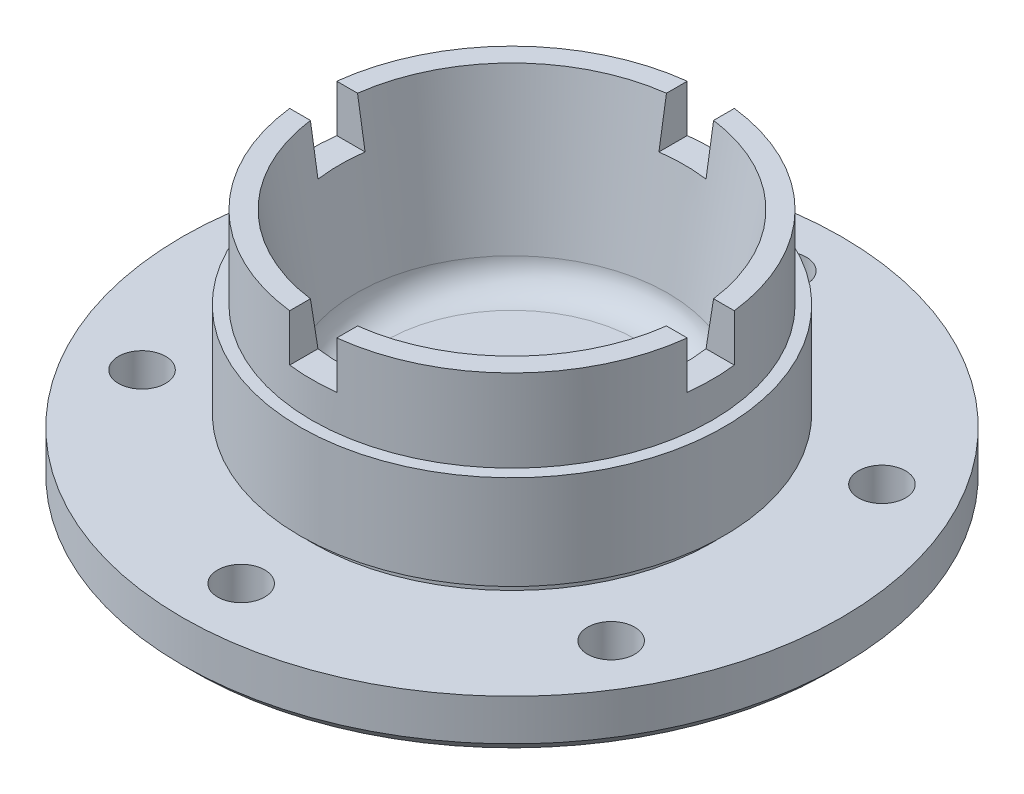
from build123d import *

# Parameters (mm, degrees)
SKETCH2_W          = 33.532576539
SKETCH2_H          = 8
SKETCH2_W_2        = 8
SKETCH2_H_2        = 33.532576539
CUT_EXTRUDE1_DEPTH = 8
SKETCH3_R          = 4
CUT_EXTRUDE2_DEPTH = 93
SCALE_1_SCALE      = 1.875


with BuildPart() as part:
    # Sketch1 → Revolve1 (revolve)
    with BuildSketch(Plane.XY, mode=Mode.PRIVATE) as revolve1_sk:
        with BuildLine():
            Line((0, 11), (0, 2))
            Line((0, 2), (31, 2))
            Line((31, 2), (32, 0))
            Line((32, 0), (54, 0))
            Line((54, 0), (56, 2))
            Line((56, 2), (56, 9))
            Line((56, 9), (34, 9))
            Line((34, 9), (34, 11))
            Line((34, 11), (36, 11))
            Line((36, 11), (36, 27))
            Line((36, 27), (34, 27))
            Line((34, 27), (34, 41))
            Line((34, 41), (30.5, 41))
            Line((30.5, 41), (26.45024814, 15.502481405))
            ThreePointArc((26.45024814, 15.502481405), (24.830088793, 12.292737332), (21.475062189, 11))
            Line((21.475062189, 11), (16.570568921, 11))
            Line((16.570568921, 11), (0, 11))
        make_face()
    revolve(revolve1_sk.sketch.rotate(Axis((0, 2, 0), (0, 1, 0)), 90), axis=Axis((0, 2, 0), (0, 1, 0)))

    # Sketch2 → Cut-Extrude1 (cut)
    with BuildSketch(Plane(origin=(0, 41, 0), x_dir=(1, 0, 0), z_dir=(0, 1, 0))):
        with Locations((31.449191607, 0)):
            Rectangle(SKETCH2_W, SKETCH2_H)
        with Locations((0, 31.449191607)):
            Rectangle(SKETCH2_W_2, SKETCH2_H_2)
        with Locations((0, -31.449191607)):
            Rectangle(SKETCH2_W_2, SKETCH2_H_2)
        with Locations((-31.449191607, 0)):
            Rectangle(SKETCH2_W, SKETCH2_H)
    extrude(amount=-CUT_EXTRUDE1_DEPTH, mode=Mode.SUBTRACT)

    # Sketch3 → Cut-Extrude2 (cut)
    with BuildSketch(Plane(origin=(0, 41, 0), x_dir=(1, 0, 0), z_dir=(0, 1, 0))):
        with Locations(Location((-39.837168574, -23, 0), (0, 0, 270))):
            Circle(SKETCH3_R)
        with Locations(Location((0, 46, 0), (0, 0, 270))):
            Circle(SKETCH3_R)
        with Locations(Location((39.837168574, 23, 0), (0, 0, 270))):
            Circle(SKETCH3_R)
        with Locations(Location((-39.837168574, 23, 0), (0, 0, 270))):
            Circle(SKETCH3_R)
        with Locations(Location((0, -46, 0), (0, 0, 270))):
            Circle(SKETCH3_R)
        with Locations(Location((39.837168574, -23, 0), (0, 0, 270))):
            Circle(SKETCH3_R)
    extrude(amount=-CUT_EXTRUDE2_DEPTH, mode=Mode.SUBTRACT)


with BuildPart() as part_1:
    # Scale 1: scaled about (0, 10.8729077, 0)
    add(part.part.scale(SCALE_1_SCALE).moved(Location((0, -9.513794238, 0))))


solid = part_1.part
